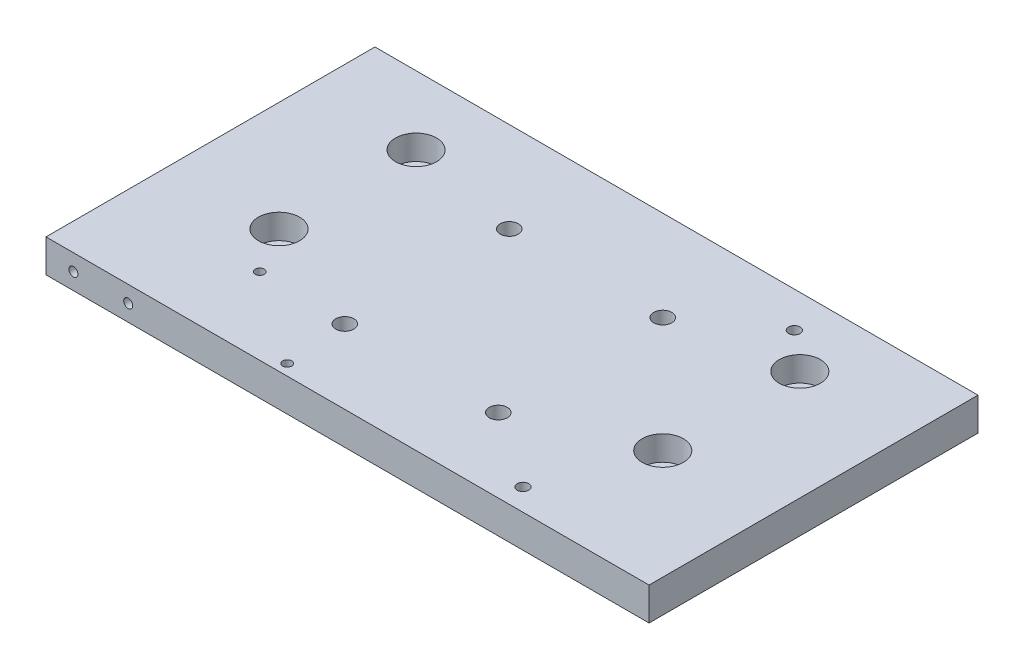
from build123d import *

# Parameters (mm, degrees)
SKETCH_1_W                  = 220
SKETCH_1_H                  = 12
EXTRUDE_1_DEPTH             = 60
HOLE_WIZARD_M6_1_D          = 5
HOLE_WIZARD_M6_1_DEPTH      = 13
HOLE_WIZARD_M6_1_TIP        = 1.502151548
HOLE_WIZARD_2_D             = 9
HOLE_WIZARD_2_CBORE_D       = 15
HOLE_WIZARD_2_CBORE_DEPTH   = 9
HOLE_WIZARD_2_2_D           = 6.6
HOLE_WIZARD_2_2_CBORE_D     = 11
HOLE_WIZARD_2_2_CBORE_DEPTH = 6.8
HOLE_WIZARD_M4_1_D          = 3.3
HOLE_WIZARD_M5_2_D          = 4.2
HOLE_WIZARD_M4_2_D          = 3.3
HOLE_WIZARD_M4_2_DEPTH      = 10.1
HOLE_WIZARD_M4_2_TIP        = 0.991420021


with BuildPart() as part:
    # 草图1 → 凸台-拉伸1 (new, symmetric)
    with BuildSketch(Plane.XY):
        Rectangle(SKETCH_1_W, SKETCH_1_H)
    extrude(amount=EXTRUDE_1_DEPTH, both=True)

    # M6 螺纹孔1
    with Locations(Plane(origin=(70, 0, -60), x_dir=(-1, 0, 0), z_dir=(0, 0, -1))):
        with Locations((0, 0), (70, 0), (140, 0)):
            Hole(HOLE_WIZARD_M6_1_D / 2, depth=HOLE_WIZARD_M6_1_DEPTH)
            with Locations((0, 0, -(HOLE_WIZARD_M6_1_DEPTH + HOLE_WIZARD_M6_1_TIP / 2))):  # 118° drill point
                Cone(0, HOLE_WIZARD_M6_1_D / 2, HOLE_WIZARD_M6_1_TIP, mode=Mode.SUBTRACT)

    # Hole Wizard 2 (through all)
    with Locations(Plane(origin=(-70, 6, -35), x_dir=(0, 0, 1), z_dir=(0, 1, 0))):
        with Locations((0, 0), (50, 0), (0, 140), (50, 140)):
            CounterBoreHole(HOLE_WIZARD_2_D / 2, HOLE_WIZARD_2_CBORE_D / 2, HOLE_WIZARD_2_CBORE_DEPTH)

    # Hole Wizard 2 2 (through all)
    with Locations(Plane(origin=(-28, -6, -27), x_dir=(0, 0, -1), z_dir=(0, -1, 0))):
        with Locations((0, 0), (0, 56), (-60, 56), (-60, 0)):
            CounterBoreHole(HOLE_WIZARD_2_2_D / 2, HOLE_WIZARD_2_2_CBORE_D / 2, HOLE_WIZARD_2_2_CBORE_DEPTH)

    # M4 螺纹孔1 (through all)
    with Locations(Plane(origin=(0, -6, 0), x_dir=(-1, 0, 0), z_dir=(0, -1, 0))):
        with Locations((26, -56), (60, -32)):
            Hole(HOLE_WIZARD_M4_1_D / 2)

    # M5 螺纹孔2 (through all)
    with Locations(Plane(origin=(0, -6, 0), x_dir=(-1, 0, 0), z_dir=(0, -1, 0))):
        with Locations((-56, -52), (-56, 47)):
            Hole(HOLE_WIZARD_M5_2_D / 2)

    # M4 螺纹孔2
    with Locations(Plane.XY.offset(60)):
        with Locations((-100, 0), (-80, 0)):
            Hole(HOLE_WIZARD_M4_2_D / 2, depth=HOLE_WIZARD_M4_2_DEPTH)
            with Locations((0, 0, -(HOLE_WIZARD_M4_2_DEPTH + HOLE_WIZARD_M4_2_TIP / 2))):  # 118° drill point
                Cone(0, HOLE_WIZARD_M4_2_D / 2, HOLE_WIZARD_M4_2_TIP, mode=Mode.SUBTRACT)


solid = part.part
